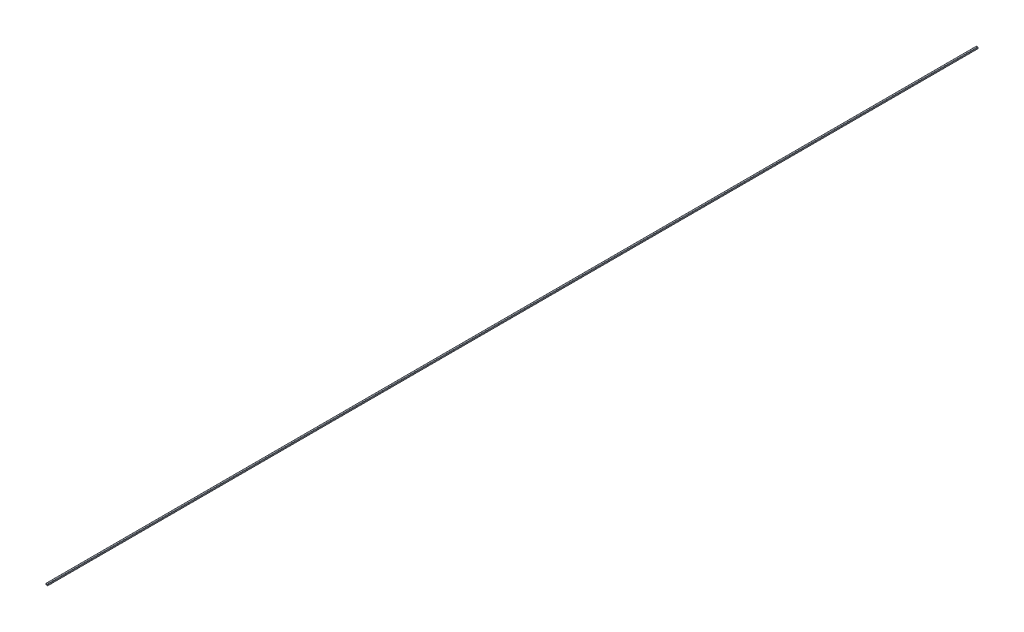
from build123d import *

# Parameters (mm, degrees)
BOSS_EXTRUDE1_DEPTH = 16840


with BuildPart() as part:
    # Sketch1 → Boss-Extrude1 (new body)
    with BuildSketch(Plane.XY):
        with BuildLine():
            Line((-10, -13.2), (-6.5, -13.2))
            Line((-6.5, -13.2), (-6.5, -15))
            Line((-6.5, -15), (-10, -15))
            ThreePointArc((-10, -15), (-14.242640687, -13.242640687), (-16, -9))
            Line((-16, -9), (-16, 9))
            ThreePointArc((-16, 9), (-14.242640687, 13.242640687), (-10, 15))
            Line((-10, 15), (10, 15))
            ThreePointArc((10, 15), (14.242640687, 13.242640687), (16, 9))
            Line((16, 9), (16, -9))
            ThreePointArc((16, -9), (14.242640687, -13.242640687), (10, -15))
            Line((10, -15), (6.5, -15))
            Line((6.5, -15), (6.5, -13.2))
            Line((6.5, -13.2), (10, -13.2))
            ThreePointArc((10, -13.2), (12.969848481, -11.969848481), (14.2, -9))
            Line((14.2, -9), (14.2, 9))
            ThreePointArc((14.2, 9), (12.969848481, 11.969848481), (10, 13.2))
            Line((10, 13.2), (-10, 13.2))
            ThreePointArc((-10, 13.2), (-12.969848481, 11.969848481), (-14.2, 9))
            Line((-14.2, 9), (-14.2, -9))
            ThreePointArc((-14.2, -9), (-12.969848481, -11.969848481), (-10, -13.2))
        make_face()
    extrude(amount=BOSS_EXTRUDE1_DEPTH)


solid = part.part
